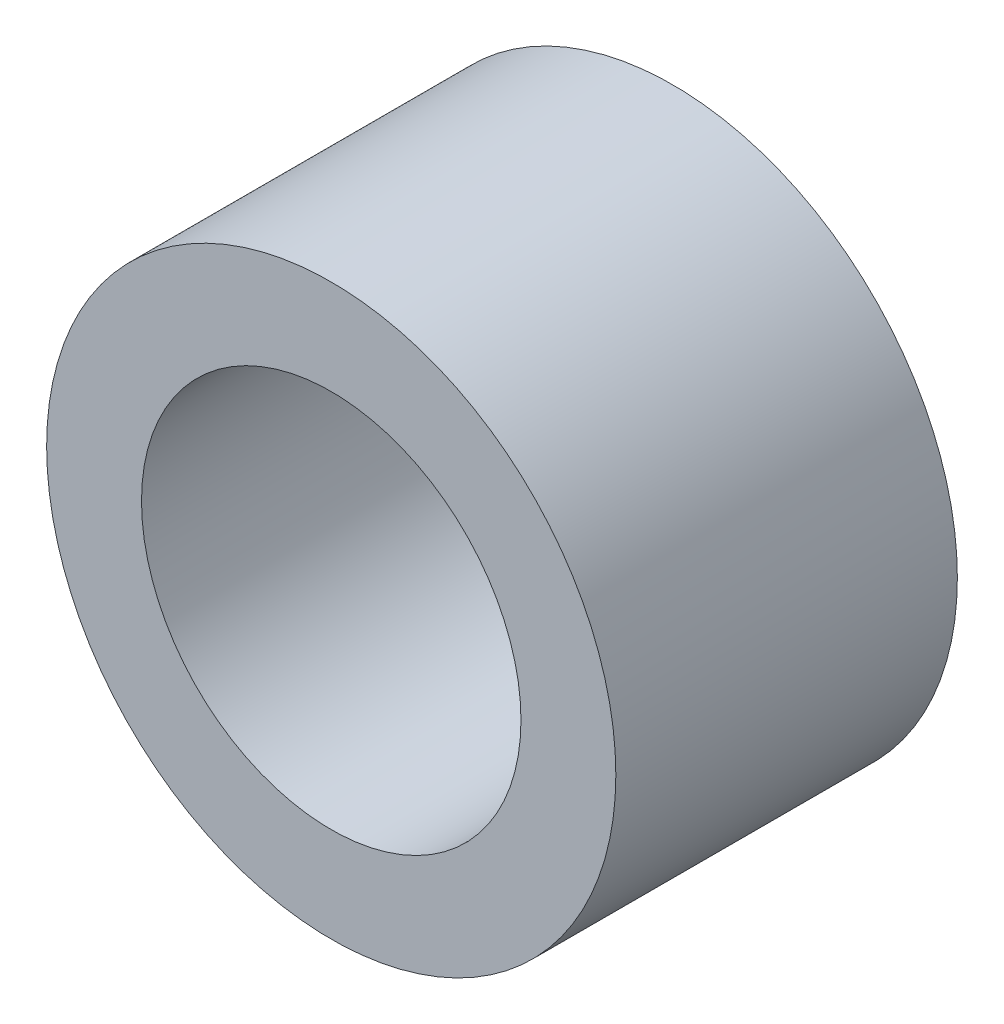
from build123d import *

# Parameters (mm, degrees)
SKETCH1_R           = 7.5
SKETCH1_R_2         = 5
BOSS_EXTRUDE1_DEPTH = 9


with BuildPart() as part:
    # Sketch1 → Boss-Extrude1 (new body)
    with BuildSketch(Plane.XY):
        Circle(SKETCH1_R)
        Circle(SKETCH1_R_2, mode=Mode.SUBTRACT)
    extrude(amount=BOSS_EXTRUDE1_DEPTH)


solid = part.part
